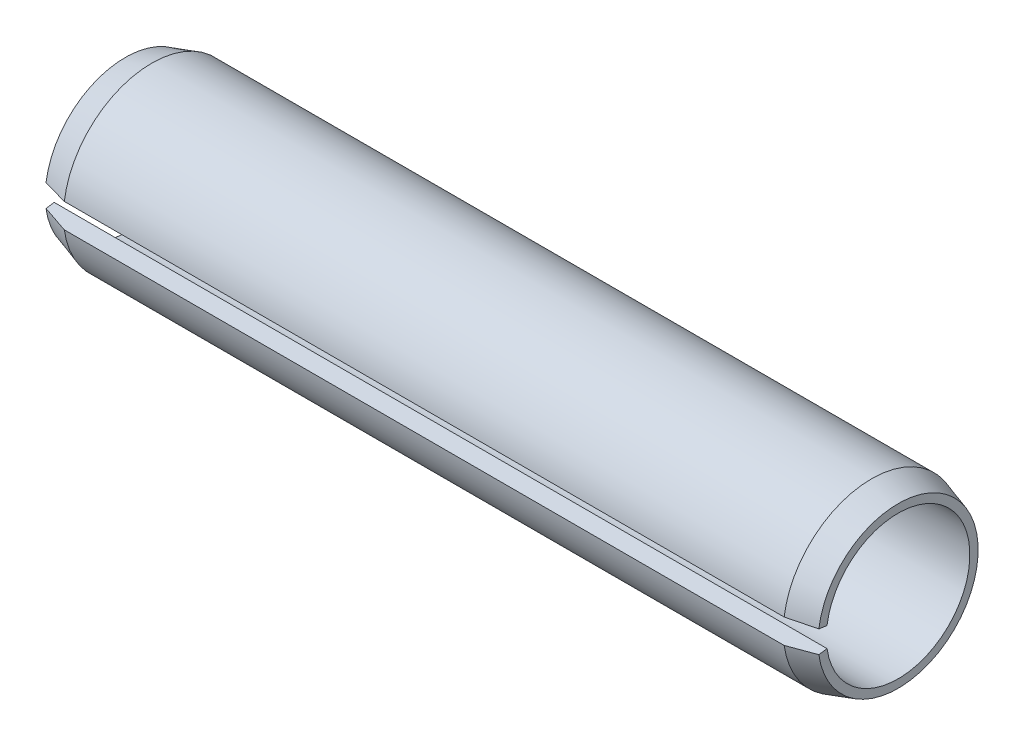
SolidWorks part; units mm, degrees
ref_plane "Front" through (0, 0, 0) normal (0, 0, 1) x (1, 0, 0)
ref_plane "Top" through (0, 0, 0) normal (0, 1, 0) x (1, 0, 0)
ref_plane "Right" through (0, 0, 0) normal (1, 0, 0) x (0, 0, -1)
other "Configuration Table"
sketch "Sketch1" plane through (0, 0, 0) normal (1, 0, 0) x (0, 0, -1)
  circle A0 centre (0, 0) radius 6.5 construction
  circle A1 centre (0, 0) radius 8
  circle A2 centre (0, 0) radius 7.25
extrude "Base-Extrude" add sketch "Sketch1" along normal blind 70
sketch "Sketch2" plane through (0, 0, 0) normal (1, 0, 0) x (0, 0, -1)
  circle A0 centre (0, 0) radius 7.25 construction
  circle A1 centre (0, 0) radius 7.25
  circle A2 centre (0, 0) radius 6.5
  circle A3 centre (0, 0) radius 6.5 construction
extrude "Extrude2" add sketch "Sketch2" along normal up to surface (70 mm away) up to face at (70, 0, -8)
sketch "Sketch3" plane through (0, 0, 0) normal (0, 0, 1) x (1, 0, 0)
  line L0 (70, 8) -> (70, 7.25)
  line L2 (70, 8) -> (67.6, 8)
  line L4 (67.6, 8) -> (70, 7.25)
  line L5 (35, 0) -> (3.6295, 0) construction
  line L7 (35, 0) -> (35, 0.7569) construction
  line L8 (2.4, 8) -> (0, 7.25)
  line L9 (0, 8) -> (2.4, 8)
  line L10 (0, 8) -> (0, 7.25)
  dimension "a" = 2.4
revolve "Cut-Revolve1" cut sketch "Sketch3" angle 360 about L5
sketch "Sketch4" plane through (0, 0, 0) normal (1, 0, 0) x (0, 0, -1)
  line L0 (0, 0) -> (-0.577, 0) construction
  line L1 (0, 0) -> (-8.1, 1.1384)
  line L2 (-8.1, 1.1384) -> (-8.1, -1.1384)
  line L3 (0, 0) -> (-8.1, -1.1384)
  circle A0 centre (0, 0) radius 8 construction
  point P2 (-8, 0)
  point P8 (-8.1, 0)
  dimension "D1" = 8
  dimension "D2" = 0.1
extrude "Gap" cut sketch "Sketch4" along normal through all
equation "\"s2@Sketch1\" = \"s1@Sketch1\" / 2"
